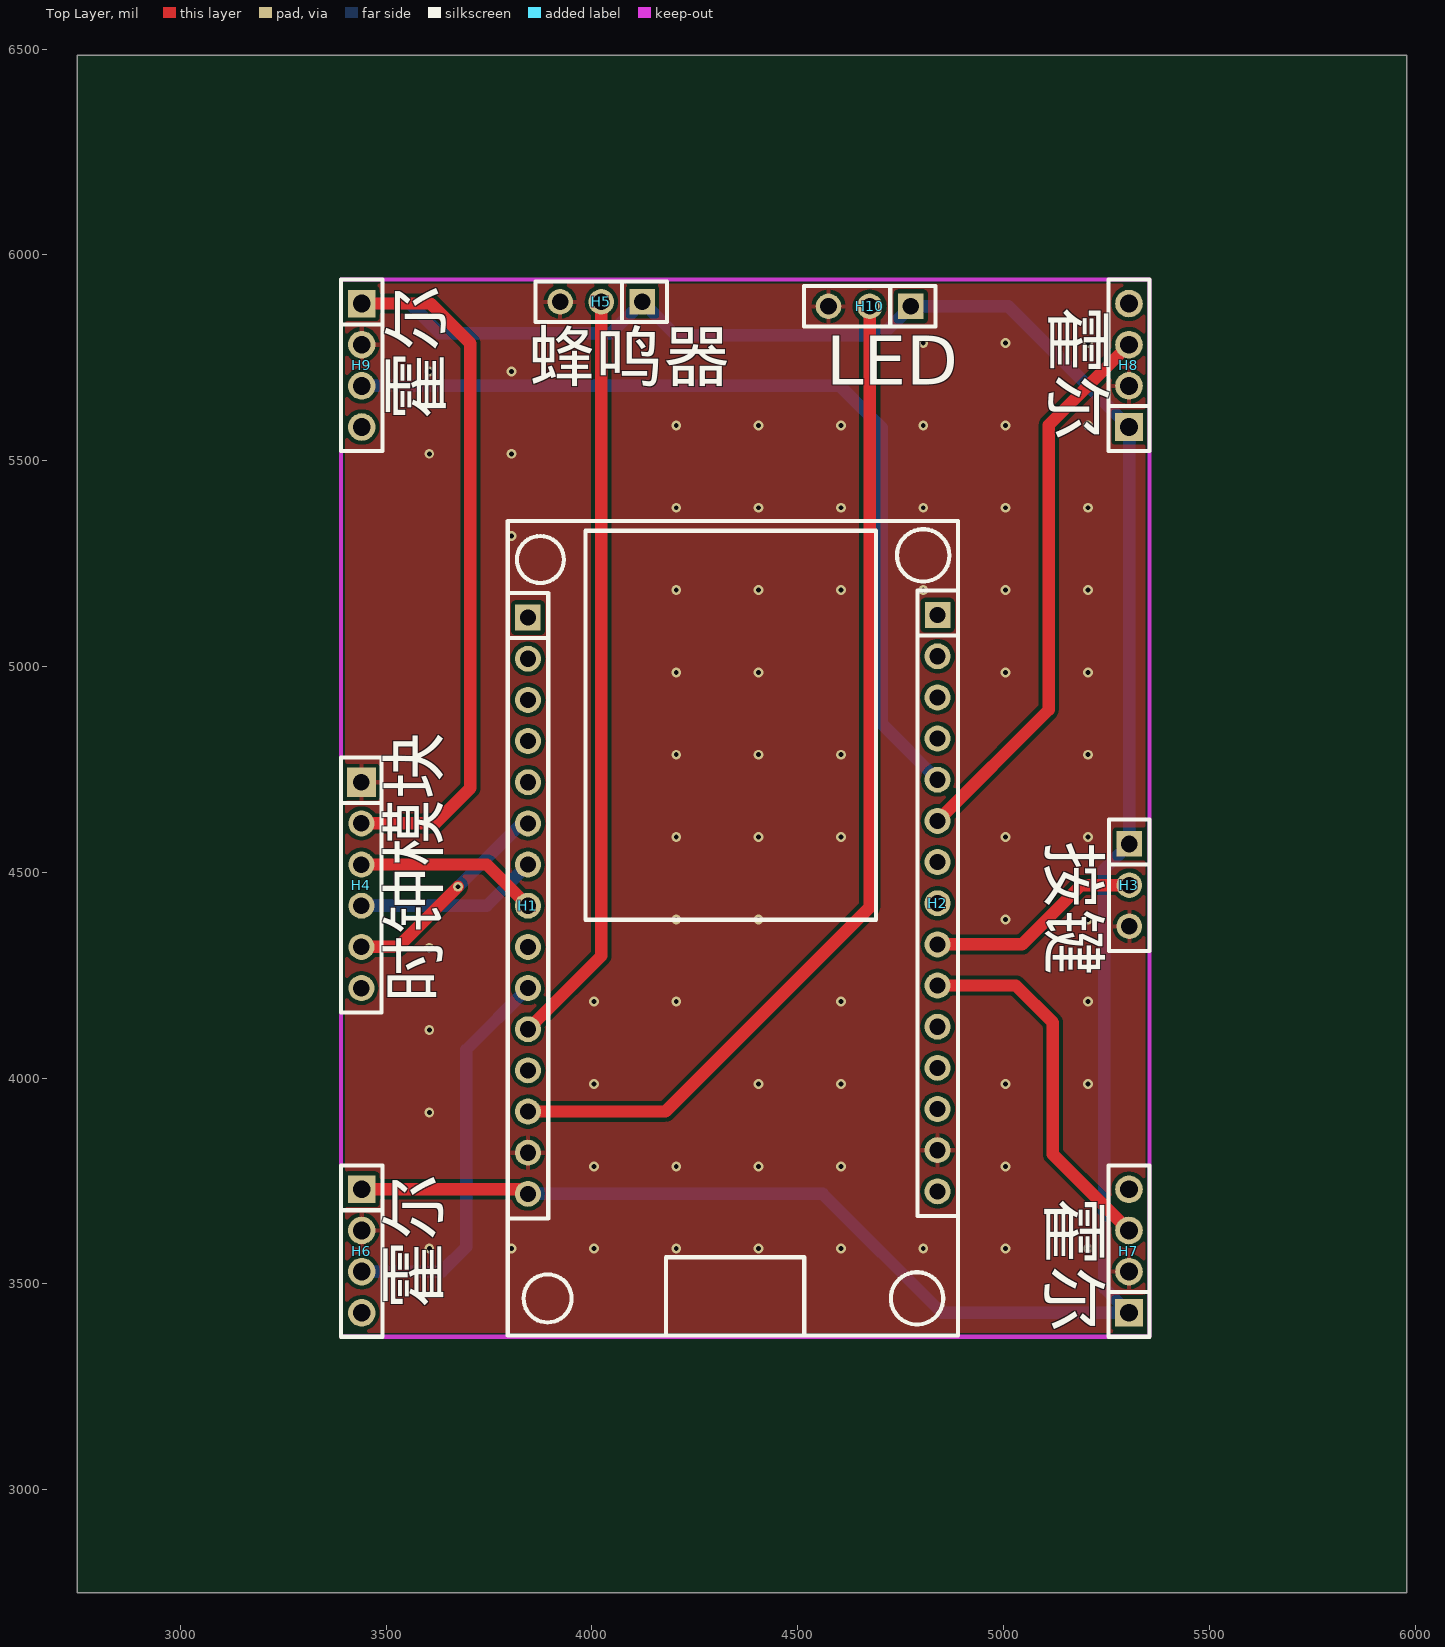
[diagram p0: Top Layer view]
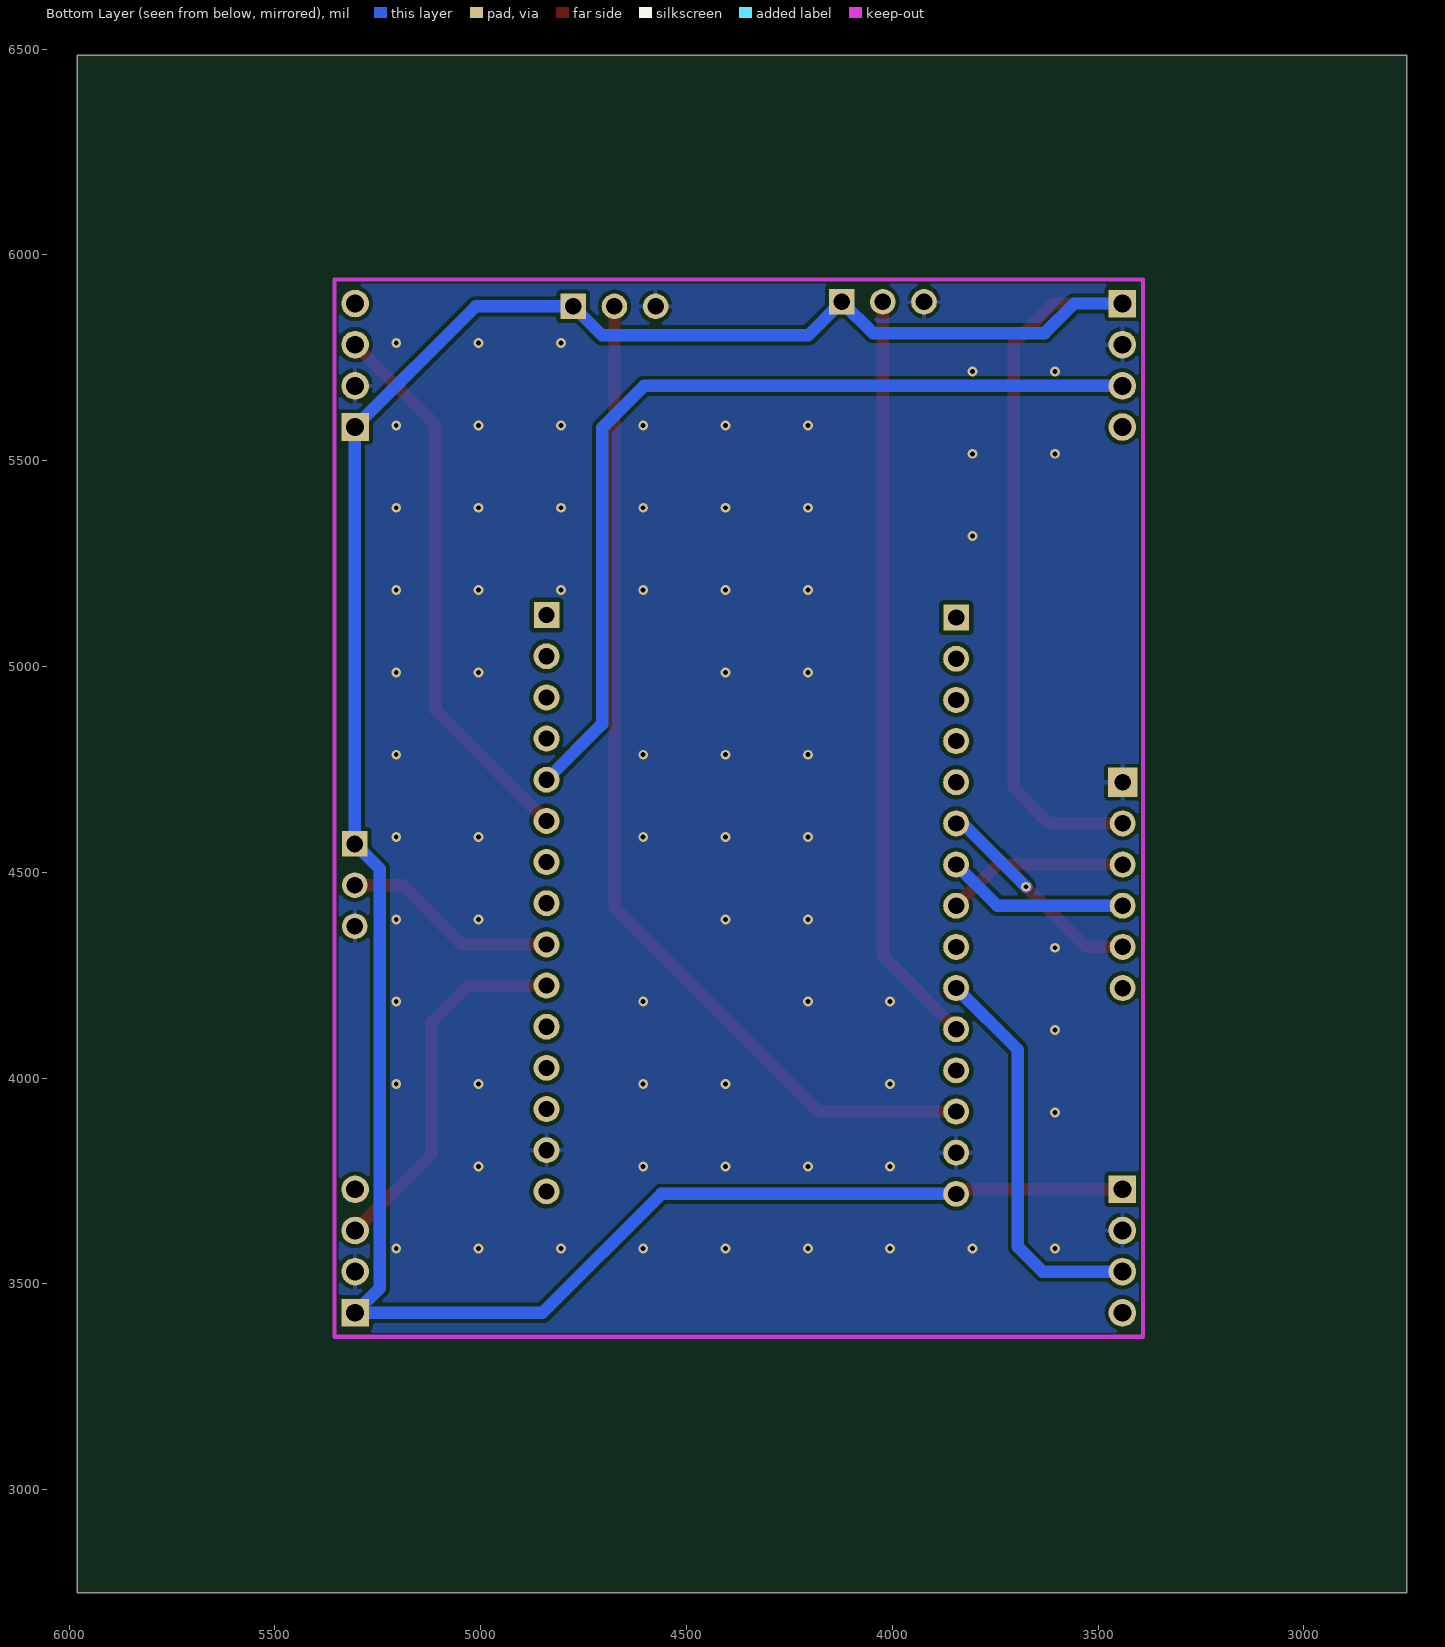
[diagram p1: Bottom Layer view, seen from below]
# Altium PCB MISC51778.pcbdoc
Units mil, origin at the board's own origin, x right, y up, seen from the top; angles counter-clockwise.
Board outline 3230 x 3735 mil, 2 copper layers (Top Layer, Bottom Layer), stack 62.206 mil thick; 10 components, 29 nets, 61 pads, 70 vias.

## Layer stack, top to bottom
Top Solder Mask Layer: solder mask 0.394, Dk 3.3
Top Layer: signal copper 1.379
Dielectric1: surface 59.449, FR4, Dk 4.5
Bottom Layer: signal copper 1.378
Bottom Solder Mask Layer: solder mask 0.394, Dk 3.3

## Board outline
5980,2750 2750,2750 2750,6485 5980,6485

## Design rules (kind name [scope] priority, off if disabled: settings)
BoardOutlineClearance copperThickness2oz_1 [All] p2 off: genericclearance=7.99 ignorepadtopadclearanceinfootprint=FALSE except(0: Arc-SplitContinuation Track-SplitContinuation SMDPad-SplitContinuation THPad-SplitContinuation Via-SplitContinuation Fill-SplitContinuation Region-SplitContinuation Poly-SplitContinuation Text-SplitContinuation Hole-SplitContinuation; 5.98: Arc-CutoutEdge SMDPad-CutoutEdge THPad-CutoutEdge Via-CutoutEdge Fill-CutoutEdge Region-CutoutEdge Text-CutoutEdge; 6.93: Hole-OutlineEdge Hole-CutoutEdge; 10: Poly-OutlineEdge Poly-CutoutEdge; 11.81: Arc-OutlineEdge Track-OutlineEdge SMDPad-OutlineEdge THPad-OutlineEdge Via-OutlineEdge Fill-OutlineEdge Region-OutlineEdge Text-OutlineEdge Track-CutoutEdge)
BoardOutlineClearance copperThickness1oz_1 [All] p4: genericclearance=4.02 ignorepadtopadclearanceinfootprint=FALSE except(0: Arc-SplitContinuation Track-SplitContinuation SMDPad-SplitContinuation THPad-SplitContinuation Via-SplitContinuation Fill-SplitContinuation Region-SplitContinuation Poly-SplitContinuation Text-SplitContinuation Hole-SplitContinuation; 6: SMDPad-CutoutEdge THPad-CutoutEdge Via-CutoutEdge Fill-CutoutEdge Region-CutoutEdge Text-CutoutEdge; 6.93: Hole-OutlineEdge Hole-CutoutEdge; 10: Poly-OutlineEdge Poly-CutoutEdge; 11.8: Arc-OutlineEdge Track-OutlineEdge SMDPad-OutlineEdge THPad-OutlineEdge Via-OutlineEdge Fill-OutlineEdge Region-OutlineEdge Text-OutlineEdge; 11.81: Arc-CutoutEdge Track-CutoutEdge)
Clearance copperThickness2oz [All] p1 off: gap=7.99 ignorepadtopadclearanceinfootprint=FALSE except(5.98: SMDPad-Track SMDPad-SMDPad THPad-Track SMDPad-THPad THPad-THPad Track-Via SMDPad-Via THPad-Via Via-Via Fill-Track Region-Track Fill-SMDPad Region-SMDPad Fill-THPad Region-THPad Fill-Via Region-Via Fill-Fill Fill-Region Region-Region Arc-Track Arc-SMDPad Arc-THPad Arc-Via Fill-Arc Region-Arc Arc-Arc Text-Track SMDPad-Text Text-THPad Text-Via Fill-Text Region-Text Arc-Text Text-Text; 6.93: Hole-Track Hole-SMDPad Hole-THPad Hole-Via Fill-Hole Region-Hole Hole-Arc Hole-Text; 10: Poly-Track Poly-SMDPad Poly-THPad Poly-Via Poly-Fill Poly-Region Poly-Poly Poly-Arc Poly-Text Poly-Hole)
Clearance copperThickness1oz [All] p3: gap=4.02 ignorepadtopadclearanceinfootprint=FALSE except(5.98: SMDPad-Track SMDPad-SMDPad THPad-Track SMDPad-THPad THPad-THPad Track-Via SMDPad-Via THPad-Via Via-Via Fill-Track Region-Track Fill-SMDPad Region-SMDPad Fill-THPad Region-THPad Fill-Via Region-Via Fill-Fill Fill-Region Region-Region; 6: Arc-Track Arc-SMDPad Arc-THPad Arc-Via Fill-Arc Region-Arc Arc-Arc Text-Track SMDPad-Text Text-THPad Text-Via Fill-Text Region-Text Arc-Text Text-Text; 6.93: Hole-Track Hole-SMDPad Hole-THPad Hole-Via Fill-Hole Region-Hole Hole-Arc Hole-Text; 10: Poly-Track Poly-SMDPad Poly-THPad Poly-Via Poly-Fill Poly-Region Poly-Poly Poly-Arc Poly-Text Poly-Hole)
DiffPairsRouting differentialPair [All] p1: maxlimit=6 minlimit=6 mostfreqgap=6 toplayer_minwidth=5 toplayer_prefwidth=10 toplayer_maxwidth=100 toplayer_mingap=6 toplayer_prefgap=6 toplayer_maxgap=6 bottomlayer_minwidth=5 bottomlayer_prefwidth=10 bottomlayer_maxwidth=100 bottomlayer_mingap=6 bottomlayer_prefgap=6 bottomlayer_maxgap=6 maxuncoupledlength=10
HoleToHoleClearance otherClearance [All] p1: gap=11.81 allowstackedmicrovias=TRUE
Length netLength [All] p1: minlimit=0 maxlimit=0
MatchedLengths netLengthTolerance [All] p1: tolerance=1000
PasteMaskExpansion pasteMaskExpansion [All] p1: expansion=0
PlaneConnect innerPlane [All] p1: planeconnectstyle=Relief reliefexpansion=20 reliefentries=4 reliefconductorwidth=10 reliefairgap=10
PolygonConnect copperRegion [(InNet('GND'))] p1: connectstyle=Relief reliefconductorwidth=10 reliefentries=4 polygonreliefangle="90 Angle" airgapwidth=10 via.connectstyle=Relief via.reliefconductorwidth=10 via.reliefentries=4 via.polygonreliefangle="90 Angle" via.airgapwidth=10
RoutingVias viaSize [All] p1: holewidth=12.01 width=24.02 viastyle="Through Hole" minholewidth=11.81 minwidth=19.68 maxholewidth=248.03 maxwidth=393.7
SolderMaskExpansion solderMaskExpansion [IsVia] p1: expansion=-1000 istentingtop=TRUE
SolderMaskExpansion solderMaskExpansion [All] p2: expansion=2 istentingtop=FALSE
Width copperThickness2oz_2 [All] p1 off: maxlimit=100 minlimit=8 preferedwidth=10
Width copperThickness1oz_2 [All] p2: maxlimit=100 minlimit=5 preferedwidth=10

## Components (designator, comment, footprint, x,y, rotation, side; value= is the part's Value field where it differs from the comment)
H1 "" HDR-TH_15P-P2.54-V-F-1 3844.84,4418.94 r270 top
H2 "" HDR-TH_15P-P2.54-V-F-1 4840,4425 r270 top
H3 "" HDR-TH_3P-P2.54-V-F 5305.79,4468.94 r270 top
H4 "" HDR-TH_6P-P2.54-V-F 3440.27,4468.94 r270 top
H5 "" HDR-TH_3P-P2.54-V-F 4023.03,5885.99 r180 top
H6 "" HDR-TH_4P-P2.54-V-F 3441.06,3580 r270 top
H7 "" HDR-TH_4P-P2.54-V-F 5305,3580 r90 top
H8 "" HDR-TH_4P-P2.54-V-F 5305,5731.93 r90 top
H9 "" HDR-TH_4P-P2.54-V-F 3441.06,5731.93 r270 top
H10 "" HDR-TH_3P-P2.54-V-F 4675,5875 r180 top

## Footprints (in the part's own frame and the unit in brackets; to place one, negate y for a bottom-side part, rotate by r counter-clockwise, add the part's x,y. Pads: shape width x height; smd on the part's side, far side on the other; paste and mask are expansions set on the pad)
HDR-TH_3P-P2.54-V-F [mil]
  rect 62x62 hole 40.16: 1(-100,0)
  round 62 hole 40.16: 2(0,0) 3(100,0)
  silkscreen extent -160,-49 160,49
HDR-TH_4P-P2.54-V-F [mm]
  rect 1.7x1.7 hole 1.1: 1(-3.81,0)
  round 1.7 hole 1.1: 2(-1.27,0) 3(1.27,0) 4(3.81,0)
  silkscreen extent -5.29,-1.27 5.29,1.27
HDR-TH_6P-P2.54-V-F [mm]
  rect 1.8x1.8 hole 1.02: 1(-6.35,0)
  round 1.6 hole 1.02: 2(-3.81,0) 3(-1.27,0) 4(1.27,0) 5(3.81,0) 6(6.35,0)
  silkscreen extent -7.87,-1.25 7.87,1.25
HDR-TH_15P-P2.54-V-F-1 [mm]
  rect 1.6x1.575 hole 1: 1(-17.78,0)
  round 1.6 hole 1: 2(-15.24,0) 3(-12.7,0) 4(-10.16,0) 5(-7.62,0) 6(-5.08,0) 7(-2.54,0) 8(0,0) 9(2.54,0) 10(5.08,0) 11(7.62,0) 12(10.16,0) 13(12.7,0) 14(15.24,0) 15(17.78,0)
  silkscreen extent -19.3,-1.25 19.3,1.25

## Via types
v1: diameter 24.02, hole 12, Top Layer to Bottom Layer, 70 vias

## Nets (pads, with @x,y where several pads share a name; then routed paths per layer and width w, separated by ;. In a path a pad name is that pad's centre, name@x,y a point inside that pad or via, vN(x,y) a via of type N, cw(c..) or ccw(c..) an arc to the next point about the centre after c; other vN are vias at no path point)
+5V: H1.15 H3.1 H4.2 H5.1 H6.1 H7.1 H8.1 H9.1 H10.1 | length 7984.1
  Top Layer w30: H4.2 3618.94,4618.94 3705,4705 3705,5785 3608.07,5881.93 H9.1 ; H6.1 3833.78,3730 H1.15
  Bottom Layer w30: H9.1 3558.07,5881.93 3630,5810 4047.05,5810 H5.1 4204.02,5805 4705,5805 H10.1 5011.93,5875 H8.1 5305.79,5581.14 H3.1 5245,4508.15 5245,3490 H7.1 4850,3430 4561.06,3718.94 H1.15
EN: H1.1
GND: H1.14 H2.14 H3.3 H4.1 H5.3 H6.2 H7.2 H8.2 H9.2 H10.3
  other v1: 3605.16,3585.83 3805.16,3585.83 4005.16,3585.83 4205.16,3585.83 4405.16,3585.83 4605.16,3585.83 4805.16,3585.83 5005.16,3585.83 5205.16,3585.83 4005.16,3785.83 4205.16,3785.83 4405.16,3785.83 4605.16,3785.83 5005.16,3785.83 3605.16,3916.87 4005.16,3985.83 4405.16,3985.83 4605.16,3985.83 5005.16,3985.83 5205.16,3985.83 3605.16,4116.87 4005.16,4185.83 4205.16,4185.83 4605.16,4185.83 5205.16,4185.83 3605.16,4316.87 4205.16,4385.83 4405.16,4385.83 5005.16,4385.83 5205.16,4385.83 4205.16,4585.83 4405.16,4585.83 4605.16,4585.83 5005.16,4585.83 5205.16,4585.83 4205.16,4785.83 4405.16,4785.83 4605.16,4785.83 5205.16,4785.83 4205.16,4985.83 4405.16,4985.83 5005.16,4985.83 5205.16,4985.83 4205.16,5185.83 4405.16,5185.83 4605.16,5185.83 4805.16,5185.83 5005.16,5185.83 5205.16,5185.83 3805.16,5316.87 4205.16,5385.83 4405.16,5385.83 4605.16,5385.83 4805.16,5385.83 5005.16,5385.83 5205.16,5385.83 3605.16,5516.87 3805.16,5516.87 4205.16,5585.83 4405.16,5585.83 4605.16,5585.83 4805.16,5585.83 5005.16,5585.83 5205.16,5585.83 3605.16,5716.87 3805.16,5716.87 4805.16,5785.83 5005.16,5785.83 5205.16,5785.83
GPIO1: H2.3
GPIO2: H2.12
GPIO3: H2.4
GPIO4: H2.11
GPIO5: H2.8
GPIO12: H1.12
GPIO13: H1.13 H10.2 | length 2495.6
  Top Layer w30: H1.13 4178.94,3918.94 4675,4415 H10.2
GPIO14: H1.11 H5.2 | length 1840.9
  Top Layer w30: H1.11 4023.03,4297.13 H5.2
GPIO15: H2.13
GPIO16: H2.10 H7.3 | length 898.9
  Top Layer w30: H2.10 5030,4225 5120,4135 5120,3815 H7.3
GPIO17: H2.9 H3.2 | length 525.4
  Top Layer w30: H2.9 5045,4325 5188.94,4468.94 H3.2
GPIO18: H2.7
GPIO19: H2.6 H8.3 | length 1349.5
  Top Layer w30: H2.6 5110,4895 5110,5586.93 H8.3
GPIO21: H2.5 H9.3 | length 2217.1
  Bottom Layer w30: H9.3 4603.07,5681.93 4705,5580 4705,4860 H2.5
GPIO22: H2.2
GPIO23: H2.1
GPIO25: H1.8 H4.3 | length 446
  Top Layer w30: H4.3 3744.84,4518.94 H1.8
GPIO26: H1.9
GPIO27: H1.10 H6.3 | length 969.8
  Bottom Layer w30: H6.3 3635,3530 3695,3590 3695,4069.1 H1.10
GPIO32: H1.6 H4.5 | length 528.8
  Top Layer w30: H4.5 3528.94,4318.94 v1(3675,4465)
  Bottom Layer w30: v1(3675,4465) 3828.94,4618.94 H1.6
GPIO33: H1.7 H4.4 | length 446
  Bottom Layer w30: H4.4 3744.84,4418.94 H1.7
GPIO34: H1.4
GPIO35: H1.5
GPIO36: H1.2
GPIO39: H1.3
VCC: H2.15
pads on no net: H4.6 H6.4 H7.4 H8.4 H9.4

## Polygon pours and split planes (outlines as drawn)
GND on Top Layer (solid, remove dead copper, pour order 0): 3020,6235 3020,3000 5700,3000 5700,6235
GND on Bottom Layer (solid, remove dead copper, pour order 2): 3000,6230 3000,3140 5730,3140 5730,6230

## Keep-outs
Board Outline Layer:
  lines w10: 3391.06,3371.73 3391.06,5940.2 5355,5940.2 5355,3371.73 3391.06,3371.73

## Silkscreen, mask and mechanical layers (free items; w line width, h text height)
Top Silkscreen Layer:
  circle w10: c3875,5260 r57.01
  circle w10: c4805,5270 r63.64
  circle w10: c4790,3465 r63.64
  circle w10: c3892.59,3465 r58.3
  lines w10: 3795.63,3375.16 3795.63,5353.78 4889.21,5353.78 4889.21,3375.16 3795.63,3375.16 ; 3985,4385 3985,5330 4690,5330 4690,4385 3985,4385 ; 4180,3375.16 4180,3565 4516.13,3565 4516.13,3375.16 4180,3375.16
  text "霍尔" at 5125,5875 h120 r270
  text "蜂鸣器" at 3845,5695 h120
  text "LED" at 4570,5685 h120
  text "霍尔" at 3630,5600 h120 r90
  text "按键" at 5115,4575 h120 r270
  text "时钟模块" at 3625,4185 h120 r90
  text "霍尔" at 5115,3710 h120 r270
  text "霍尔" at 3625,3440 h120 r90